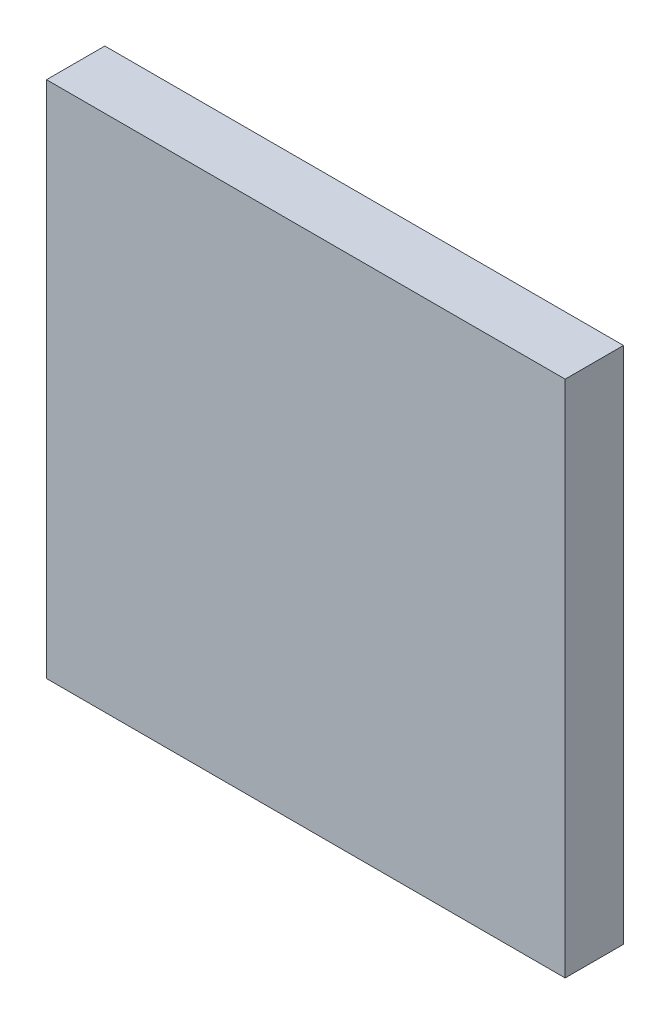
SolidWorks part; units mm, degrees
material "普通碳钢"
ref_plane "Front Plane" through (0, 0, 0) normal (0, 0, 1) x (1, 0, 0)
ref_plane "Top Plane" through (0, 0, 0) normal (0, 1, 0) x (1, 0, 0)
ref_plane "Right Plane" through (0, 0, 0) normal (1, 0, 0) x (0, 0, -1)
sketch "Sketch1" plane through (0, 0, 0) normal (0, 0, 1) x (1, 0, 0)
  line L1 (-44.45, 44.45) -> (44.45, 44.45)
  line L2 (-44.45, 44.45) -> (-44.45, -44.45)
  line L3 (-44.45, -44.45) -> (44.45, -44.45)
  line L4 (44.45, 44.45) -> (44.45, -44.45)
  dimension "D1" = 88.9
  dimension "D2" = 88.9
  dimension "D3" = 44.45
  dimension "D4" = 44.45
extrude "Boss-Extrude1" add sketch "Sketch1" along normal mid plane 10
